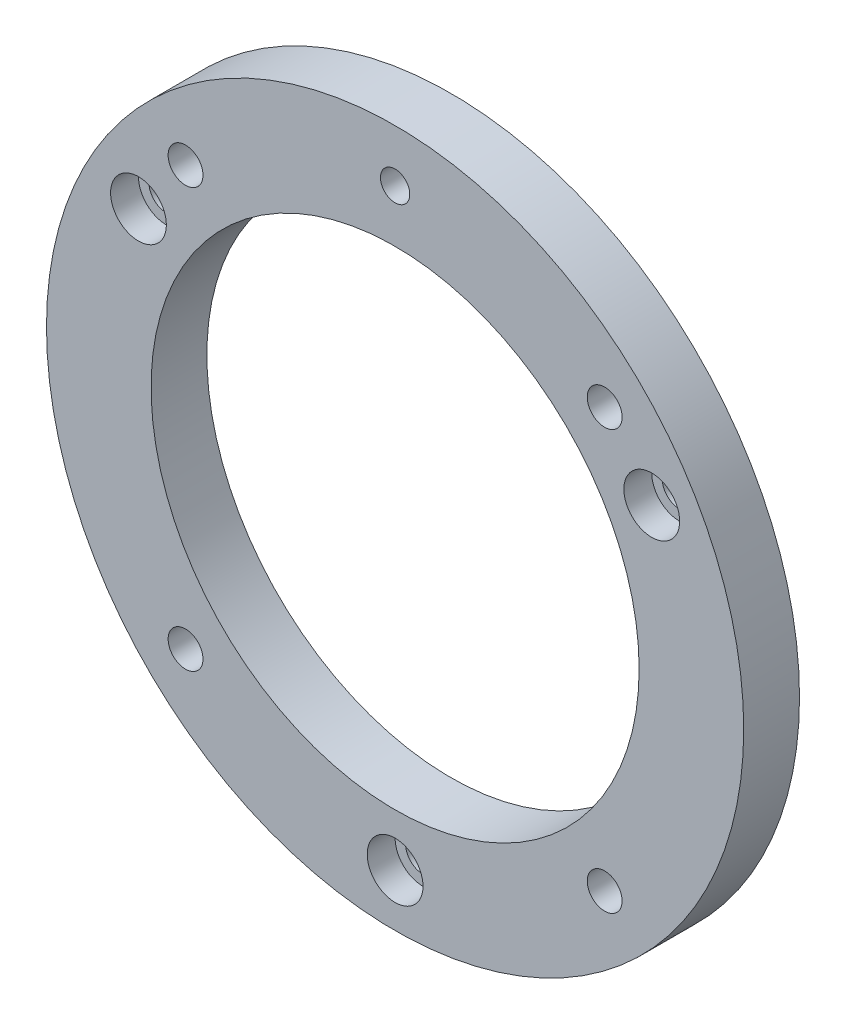
SolidWorks part; units mm, degrees
material "1060-H12 bar (SS)"
ref_plane "Front Plane" through (0, 0, 0) normal (0, 0, 1) x (1, 0, 0)
ref_plane "Top Plane" through (0, 0, 0) normal (0, 1, 0) x (1, 0, 0)
ref_plane "Right Plane" through (0, 0, 0) normal (1, 0, 0) x (0, 0, -1)
sketch "Sketch1" plane through (0, 0, 0) normal (0, 0, 1) x (1, 0, 0)
  circle A0 centre (0, 0) radius 50
extrude "Boss-Extrude1" add sketch "Sketch1" along normal blind 8
sketch "Sketch2" plane through (0, 0, 8) normal (0, 0, 1) x (1, 0, 0)
  line L0 (-50, 0) -> (50, 0) construction
  line L1 (0, 50) -> (0, -50) construction
  line L2 (-53.9261, 30.05) -> (53.7661, 30.05) construction
  line L3 (-54.8863, -30.05) -> (67.6877, -30.05) construction
  circle A0 centre (0, 0) radius 50 construction
  circle A1 centre (0, 0) radius 42.5 construction
  circle A2 centre (-30.0541, 30.05) radius 2.5
  circle A3 centre (30.0541, 30.05) radius 2.5
  circle A4 centre (-30.0541, -30.05) radius 2.5
  circle A5 centre (30.0541, -30.05) radius 2.5
  dimension "D1" = 30.05
  dimension "D3" = 5
  dimension "D4" = 5
  dimension "D5" = 5
  dimension "D6" = 5
  dimension "D2" = 30.05
extrude "Cut-Extrude1" cut sketch "Sketch2" against normal blind 8
sketch "Sketch3" plane through (0, 0, 8) normal (0, 0, 1) x (1, 0, 0)
  circle A0 centre (0, 0) radius 42.5 construction
  circle A1 centre (0, 42.5) radius 2.1
  dimension "D1" = 4.2
extrude "Cut-Extrude2" cut sketch "Sketch3" against normal blind 8
sketch "Sketch4" plane through (0, 0, 8) normal (0, 0, 1) x (1, 0, 0)
  circle A0 centre (0, 0) radius 42.5 construction
  circle A1 centre (0, -42.5) radius 4
  circle A2 centre (-36.8061, 21.25) radius 4
  circle A3 centre (36.8061, 21.25) radius 4
  point P13 (0, 0)
  dimension "D1" = 3
extrude "Cut-Extrude3" cut sketch "Sketch4" against normal blind 4
sketch "Sketch5" plane through (0, 0, 4) normal (0, 0, 1) x (1, 0, 0)
  circle A0 centre (-36.8061, 21.25) radius 2.5
  circle A1 centre (0, -42.5) radius 2.5
  circle A2 centre (36.8061, 21.25) radius 2.5
extrude "Cut-Extrude4" cut sketch "Sketch5" against normal blind 4
sketch "Sketch6" plane through (0, 0, 8) normal (0, 0, 1) x (1, 0, 0)
  circle A0 centre (0, 0) radius 35
extrude "Cut-Extrude5" cut sketch "Sketch6" against normal blind 10
